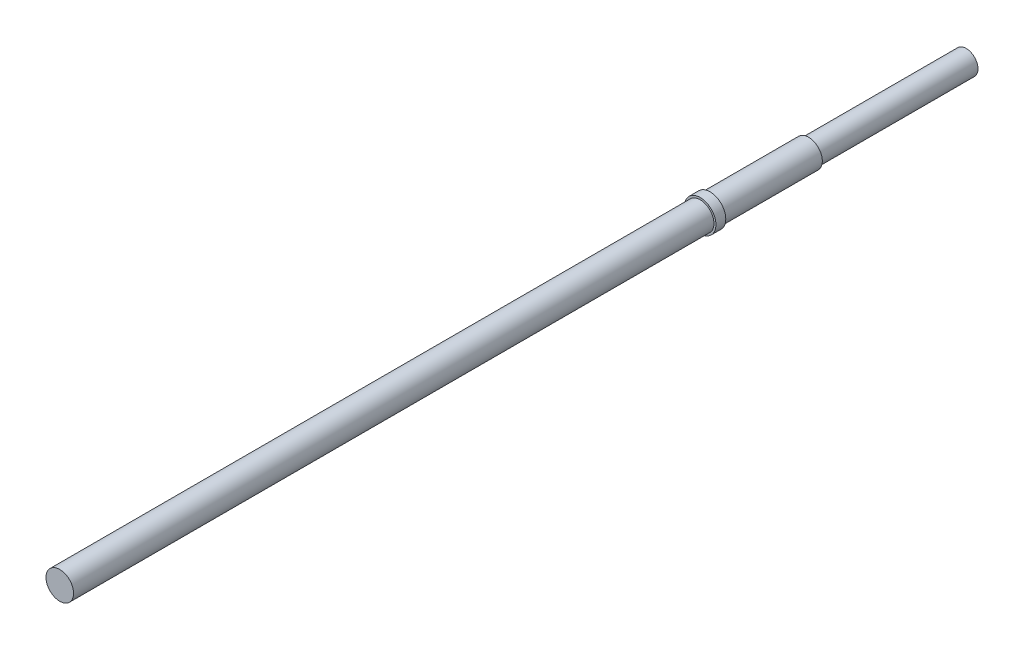
from build123d import *

# Parameters (mm, degrees)
SKETCH_1_R      = 6
EXTRUDE_1_DEPTH = 80
SKETCH_3_R      = 7
EXTRUDE_2_DEPTH = 380
EXTRUDE_START   = -330
SKETCH_4_R      = 8
EXTRUDE_3_DEPTH = 5


with BuildPart() as part:
    # 草图1 → 凸台-拉伸1 (new body)
    with BuildSketch(Plane.XY):
        Circle(SKETCH_1_R)
    extrude(amount=EXTRUDE_1_DEPTH)

    # 草图3 → 凸台-拉伸2 (add)
    with BuildSketch(Plane.XY.offset(80)):
        Circle(SKETCH_3_R)
    extrude(amount=EXTRUDE_2_DEPTH)

    # 草图4 → 凸台-拉伸3 (add)
    with BuildSketch(Plane.XY.offset(460).offset(EXTRUDE_START)):
        Circle(SKETCH_4_R)
    extrude(amount=EXTRUDE_3_DEPTH)


solid = part.part
